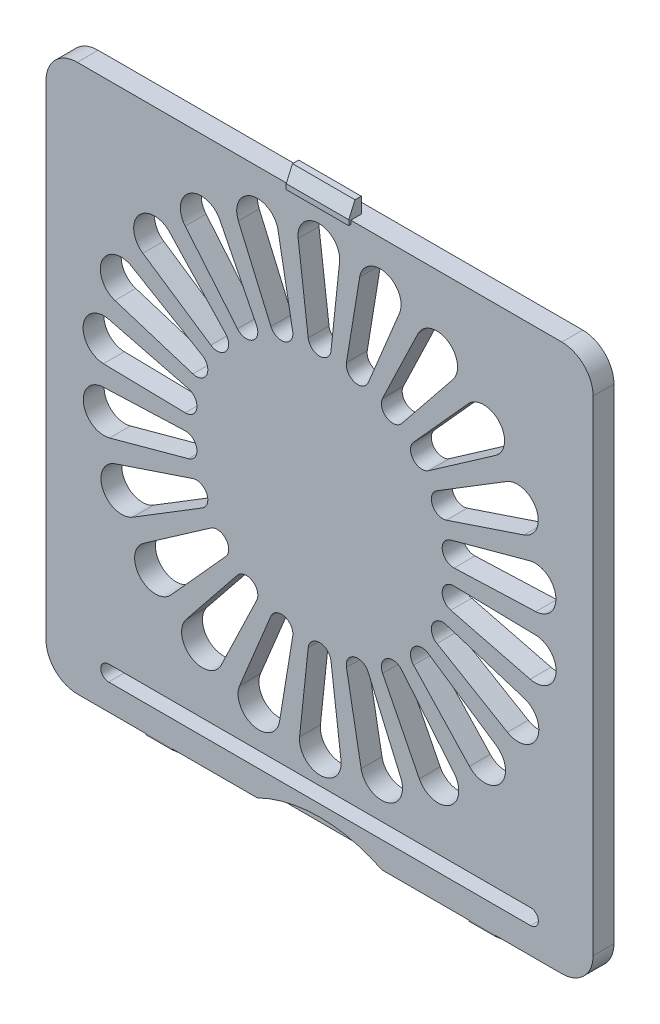
SolidWorks part; units mm, degrees
ref_plane "Front Plane" through (0, 0, 0) normal (0, 0, 1) x (1, 0, 0)
ref_plane "Top Plane" through (0, 0, 0) normal (0, 1, 0) x (1, 0, 0)
ref_plane "Right Plane" through (0, 0, 0) normal (1, 0, 0) x (0, 0, -1)
other "Configuration Table"
sketch "Sketch1" plane through (0, 0, 0) normal (0, 0, 1) x (1, 0, 0)
  line L1 (-23.25, 26.25) -> (23.25, 26.25)
  line L2 (-26.25, 23.25) -> (-26.25, -23.25)
  line L3 (-23.25, -26.25) -> (23.25, -26.25)
  line L4 (26.25, 23.25) -> (26.25, -23.25)
  line L5 (-26.25, 26.25) -> (26.25, -26.25) construction
  line L6 (-26.25, -26.25) -> (26.25, 26.25) construction
  line L11 (-20, -20) -> (20, 20) construction
  line L12 (-20, 20) -> (20, -20) construction
  arc A4 (23.25, -26.25) -> (26.25, -23.25) centre (23.25, -23.25) ccw
  arc A5 (-26.25, -23.25) -> (-23.25, -26.25) centre (-23.25, -23.25) ccw
  arc A6 (-23.25, 26.25) -> (-26.25, 23.25) centre (-23.25, 23.25) ccw
  arc A7 (23.25, 26.25) -> (26.25, 23.25) centre (23.25, 23.25) cw
  point P0 (0, 0)
  point P6 (0, 0)
  dimension "D6" = 3
  dimension "D1" = 52.5
  dimension "D2" = 52.5
extrude "Boss-Extrude1" add sketch "Sketch1" along normal blind 2
sketch "Sketch2" plane through (0, 0, 2) normal (0, 0, 1) x (1, 0, 0)
  line L6 (-20.25, -23) -> (20.25, -23) construction
  line L7 (-20.25, -22.25) -> (20.25, -22.25)
  line L8 (-20.25, -23.75) -> (20.25, -23.75)
  line L9 (26.25, -23.25) -> (26.25, 23.25) construction
  line L10 (-26.25, 23.25) -> (-26.25, -23.25) construction
  line L11 (-23.25, -26.25) -> (23.25, -26.25) construction
  line L12 (-2.0553, 22.2044) -> (-1.0917, 14.4149)
  line L13 (1.9185, 22.2399) -> (1.0939, 14.4344)
  line L14 (23.25, 26.25) -> (-23.25, 26.25) construction
  line L15 (3.847, 21.9469) -> (2.577, 14.2014)
  line L16 (7.6698, 20.8613) -> (4.6796, 13.6043)
  line L17 (9.4376, 20.0368) -> (6.0369, 12.9629)
  line L18 (12.7997, 17.9182) -> (7.8861, 11.7977)
  line L19 (14.2636, 16.6291) -> (9.0078, 10.7998)
  line L20 (16.8927, 13.6491) -> (10.4538, 9.1608)
  line L21 (17.9341, 11.9998) -> (11.2489, 7.8873)
  line L22 (19.6171, 8.3998) -> (12.1745, 5.9073)
  line L23 (20.1517, 6.5238) -> (12.5786, 4.4614)
  line L24 (20.7523, 2.5955) -> (12.909, 2.3009)
  line L25 (20.7367, 0.645) -> (12.8894, 0.7997)
  line L26 (20.2063, -3.2934) -> (12.5976, -1.3664)
  line L27 (19.6418, -5.1606) -> (12.1559, -2.8013)
  line L28 (18.0232, -8.79) -> (11.2657, -4.7974)
  line L29 (16.9555, -10.4225) -> (10.4376, -6.0497)
  line L30 (14.38, -13.4489) -> (9.021, -7.7142)
  line L31 (12.8957, -14.7144) -> (7.8737, -8.6825)
  line L32 (9.5719, -16.8926) -> (6.0456, -9.8805)
  line L33 (7.7911, -17.6887) -> (4.6719, -10.4863)
  line L34 (3.9883, -18.8423) -> (2.5804, -11.1207)
  line L35 (2.0553, -19.1044) -> (1.0917, -11.3149)
  line L36 (-1.9185, -19.1399) -> (-1.0939, -11.3344)
  line L37 (-3.847, -18.8469) -> (-2.577, -11.1014)
  line L38 (-7.6698, -17.7613) -> (-4.6796, -10.5043)
  line L39 (-9.4376, -16.9368) -> (-6.0369, -9.8629)
  line L40 (-12.7997, -14.8182) -> (-7.8861, -8.6977)
  line L41 (-14.2636, -13.5291) -> (-9.0078, -7.6998)
  line L42 (-16.8927, -10.5491) -> (-10.4538, -6.0608)
  line L43 (-17.9341, -8.8998) -> (-11.2489, -4.7873)
  line L44 (-19.6171, -5.2998) -> (-12.1745, -2.8073)
  line L45 (-20.1517, -3.4238) -> (-12.5786, -1.3614)
  line L46 (-20.7523, 0.5045) -> (-12.909, 0.7991)
  line L47 (-20.7367, 2.455) -> (-12.8894, 2.3003)
  line L48 (-20.2063, 6.3934) -> (-12.5976, 4.4664)
  line L49 (-19.6418, 8.2606) -> (-12.1559, 5.9013)
  line L50 (-18.0232, 11.89) -> (-11.2657, 7.8974)
  line L51 (-16.9555, 13.5225) -> (-10.4376, 9.1497)
  line L52 (-14.38, 16.5489) -> (-9.021, 10.8142)
  line L53 (-12.8957, 17.8144) -> (-7.8737, 11.7825)
  line L54 (-9.5719, 19.9926) -> (-6.0456, 12.9805)
  line L55 (-7.7911, 20.7887) -> (-4.6719, 13.5863)
  line L56 (-3.9883, 21.9423) -> (-2.5804, 14.2207)
  arc A6 (-20.25, -22.25) -> (-20.25, -23.75) centre (-20.25, -23) ccw
  arc A7 (20.25, -23.75) -> (20.25, -22.25) centre (20.25, -23) ccw
  circle A8 centre (0, 1.55) radius 13 construction
  arc A9 (-1.0917, 14.4149) -> (1.0939, 14.4344) centre (0, 14.55) ccw
  arc A10 (1.9185, 22.2399) -> (-2.0553, 22.2044) centre (-0.0705, 22.45) ccw
  arc A11 (7.6698, 20.8613) -> (3.847, 21.9469) centre (5.8206, 21.6233) ccw
  arc A12 (2.577, 14.2014) -> (4.6796, 13.6043) centre (3.6625, 14.0234) ccw
  arc A13 (12.7997, 17.9182) -> (9.4376, 20.0368) centre (11.2401, 19.1703) ccw
  arc A14 (6.0369, 12.9629) -> (7.8861, 11.7977) centre (7.0283, 12.4863) ccw
  arc A15 (16.8927, 13.6491) -> (14.2636, 16.6291) centre (15.749, 15.2898) ccw
  arc A16 (9.0078, 10.7998) -> (10.4538, 9.1608) centre (9.8247, 10.0632) ccw
  arc A17 (19.6171, 8.3998) -> (17.9341, 11.9998) centre (18.982, 10.2963) ccw
  arc A18 (11.2489, 7.8873) -> (12.1745, 5.9073) centre (11.8252, 6.9504) ccw
  arc A19 (20.7523, 2.5955) -> (20.1517, 6.5238) centre (20.6772, 4.5941) ccw
  arc A20 (12.5786, 4.4614) -> (12.909, 2.3009) centre (12.8677, 3.4001) ccw
  arc A21 (20.2063, -3.2934) -> (20.7367, 0.645) centre (20.6973, -1.3546) ccw
  arc A22 (12.8894, 0.7997) -> (12.5976, -1.3664) centre (12.8677, -0.3001) ccw
  arc A23 (18.0232, -8.79) -> (19.6418, -5.1606) centre (19.0406, -7.0681) ccw
  arc A24 (12.1559, -2.8013) -> (11.2657, -4.7974) centre (11.8252, -3.8504) ccw
  arc A25 (14.38, -13.4489) -> (16.9555, -10.4225) centre (15.8413, -12.0833) ccw
  arc A26 (10.4376, -6.0497) -> (9.021, -7.7142) centre (9.8247, -6.9632) ccw
  arc A27 (9.5719, -16.8926) -> (12.8957, -14.7144) centre (11.3587, -15.9941) ccw
  arc A28 (7.8737, -8.6825) -> (6.0456, -9.8805) centre (7.0283, -9.3863) ccw
  arc A29 (3.9883, -18.8423) -> (7.7911, -17.6887) centre (5.9558, -18.4836) ccw
  arc A30 (4.6719, -10.4863) -> (2.5804, -11.1207) centre (3.6625, -10.9234) ccw
  arc A31 (-1.9185, -19.1399) -> (2.0553, -19.1044) centre (0.0705, -19.35) ccw
  arc A32 (1.0917, -11.3149) -> (-1.0939, -11.3344) centre (0, -11.45) ccw
  arc A33 (-7.6698, -17.7613) -> (-3.847, -18.8469) centre (-5.8206, -18.5233) ccw
  arc A34 (-2.577, -11.1014) -> (-4.6796, -10.5043) centre (-3.6625, -10.9234) ccw
  arc A35 (-12.7997, -14.8182) -> (-9.4376, -16.9368) centre (-11.2401, -16.0703) ccw
  arc A36 (-6.0369, -9.8629) -> (-7.8861, -8.6977) centre (-7.0283, -9.3863) ccw
  arc A37 (-16.8927, -10.5491) -> (-14.2636, -13.5291) centre (-15.749, -12.1898) ccw
  arc A38 (-9.0078, -7.6998) -> (-10.4538, -6.0608) centre (-9.8247, -6.9632) ccw
  arc A39 (-19.6171, -5.2998) -> (-17.9341, -8.8998) centre (-18.982, -7.1963) ccw
  arc A40 (-11.2489, -4.7873) -> (-12.1745, -2.8073) centre (-11.8252, -3.8504) ccw
  arc A41 (-20.7523, 0.5045) -> (-20.1517, -3.4238) centre (-20.6772, -1.4941) ccw
  arc A42 (-12.5786, -1.3614) -> (-12.909, 0.7991) centre (-12.8677, -0.3001) ccw
  arc A43 (-20.2063, 6.3934) -> (-20.7367, 2.455) centre (-20.6973, 4.4546) ccw
  arc A44 (-12.8894, 2.3003) -> (-12.5976, 4.4664) centre (-12.8677, 3.4001) ccw
  arc A45 (-18.0232, 11.89) -> (-19.6418, 8.2606) centre (-19.0406, 10.1681) ccw
  arc A46 (-12.1559, 5.9013) -> (-11.2657, 7.8974) centre (-11.8252, 6.9504) ccw
  arc A47 (-14.38, 16.5489) -> (-16.9555, 13.5225) centre (-15.8413, 15.1833) ccw
  arc A48 (-10.4376, 9.1497) -> (-9.021, 10.8142) centre (-9.8247, 10.0632) ccw
  arc A49 (-9.5719, 19.9926) -> (-12.8957, 17.8144) centre (-11.3587, 19.0941) ccw
  arc A50 (-7.8737, 11.7825) -> (-6.0456, 12.9805) centre (-7.0283, 12.4863) ccw
  arc A51 (-3.9883, 21.9423) -> (-7.7911, 20.7887) centre (-5.9558, 21.5836) ccw
  arc A52 (-4.6719, 13.5863) -> (-2.5804, 14.2207) centre (-3.6625, 14.0234) ccw
  point P5 (0, -23)
  dimension "D4" = 6
  dimension "D5" = 6
  dimension "D8" = 24.7
  dimension "D9" = 3.8
  dimension "D1" = 26
  dimension "D2" = 2.2
  dimension "D3" = 4
  dimension "D6" = 1.5
  dimension "D7" = 2.5
  dimension "D10" = 22
extrude "Cut-Extrude1" cut sketch "Sketch2" against normal blind 12
sketch "Sketch3" plane through (0, 0, 0) normal (0, 0, -1) x (-1, 0, 0)
  circle A0 centre (0, -38.353) radius 13.5
  dimension "D1" = 27
extrude "Cut-Extrude2" cut sketch "Sketch3" against normal blind 1 from offset 1 offset against normal yes
sketch "Sketch4" plane through (0, 0, 0) normal (1, 0, 0) x (0, 0, -1)
  line L0 (-1, -26.25) -> (-1, -27)
  line L1 (-2, -26.25) -> (0, -26.25) construction
  line L3 (-1.8923, -26.45) -> (-1.8923, -26.25)
  line L4 (-1.8923, -26.25) -> (-1, -26.25)
  line L5 (-1, -27) -> (-1.25, -27)
  line L6 (-1.25, -27) -> (-1.8923, -26.45)
  dimension "D1" = 0.75
  dimension "D2" = 0.2
  dimension "D3" = 0.25
extrude "Boss-Extrude2" add sketch "Sketch4" along normal blind 2.5 from offset 14.25
mirror "Mirror3" about plane through (0, 0, 0) normal (1, 0, 0) of "Boss-Extrude2"
sketch "Sketch5" plane through (0, 0, 0) normal (1, 0, 0) x (0, 0, -1)
  line L0 (-1, 26.25) -> (-1, 27.75)
  line L1 (-2, 26.25) -> (0, 26.25) construction
  line L2 (-1, 27.75) -> (-1.6, 27.75)
  line L3 (-1.6, 27.75) -> (-2.2, 26.392)
  line L4 (-2.2, 26.392) -> (-2.2, 25.892)
  line L5 (-2.2, 25.892) -> (-1, 25.892)
  line L6 (-1, 25.892) -> (-1, 26.25)
  line L7 (-2, 26.25) -> (-2, 23.25) construction
  dimension "D1" = 1.5
  dimension "D2" = 0.6
  dimension "D3" = 0.5
  dimension "D4" = 0.2
extrude "Boss-Extrude3" add sketch "Sketch5" along normal mid plane 6
